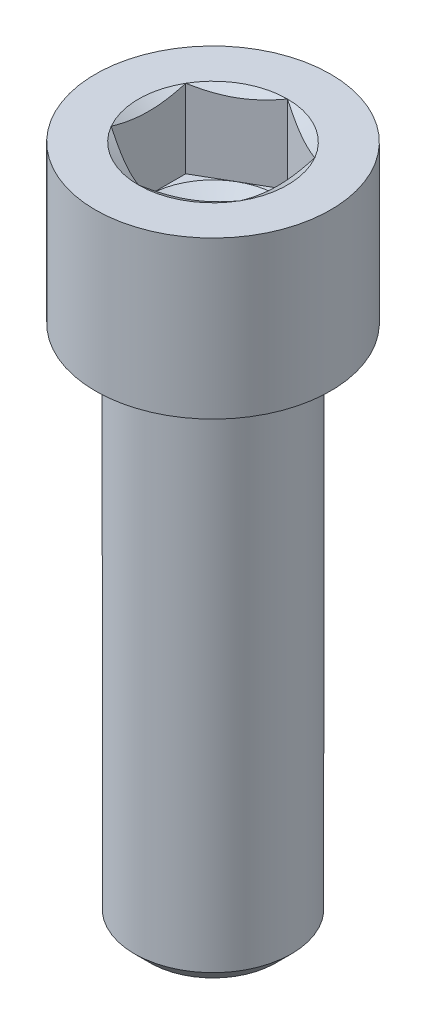
from build123d import *

# Parameters (mm, degrees)
SKETCH1_R           = 9
BOSS_EXTRUDE1_DEPTH = 12
SKETCH2_R           = 6
BOSS_EXTRUDE2_DEPTH = 40
CUT_EXTRUDE1_DEPTH  = 6
CHAMFER1_SIZE       = 1.2


with BuildPart() as part:
    # Sketch1 → Boss-Extrude1 (new body)
    with BuildSketch(Plane(origin=(0, 0, 0), x_dir=(1, 0, 0), z_dir=(0, 1, 0))):
        with Locations(Location((0, 0, 0), (0, 0, 270))):
            Circle(SKETCH1_R)
    extrude(amount=BOSS_EXTRUDE1_DEPTH)

    # Sketch2 → Boss-Extrude2 (add)
    with BuildSketch(Plane.XZ):
        with Locations(Location((0, 0, 0), (0, 0, 90))):
            Circle(SKETCH2_R)
    extrude(amount=BOSS_EXTRUDE2_DEPTH)

    # Sketch3 → Cut-Extrude1 (cut)
    with BuildSketch(Plane(origin=(0, 12, 0), x_dir=(1, 0, 0), z_dir=(0, 1, 0))):
        Polygon((0, 5.7), (-4.936344802, 2.85), (-4.936344802, -2.85), (0, -5.7), (4.936344802, -2.85), (4.936344802, 2.85), align=None)
    extrude(amount=-CUT_EXTRUDE1_DEPTH, mode=Mode.SUBTRACT)

    # Sketch4 → Cut-Revolve1 (revolve, cut)
    with BuildSketch(Plane.XY, mode=Mode.PRIVATE) as cut_revolve1_sk:
        Polygon((0, 6), (4.936344802, 6), (0, 3.15), align=None)
        Polygon((4.936344802, 11.559103466), (4.936344802, 12), (5.7, 12), align=None)
    revolve(cut_revolve1_sk.sketch.rotate(Axis((0, -3.932195077, 0), (0, 1, 0)), 270), axis=Axis((0, -3.932195077, 0), (0, 1, 0)), mode=Mode.SUBTRACT)

    # Chamfer1
    chamfer1_edges = [part.edges().sort_by_distance(p)[0] for p in [
        (0, -40, -6),
    ]]
    chamfer(chamfer1_edges, length=CHAMFER1_SIZE)


solid = part.part
